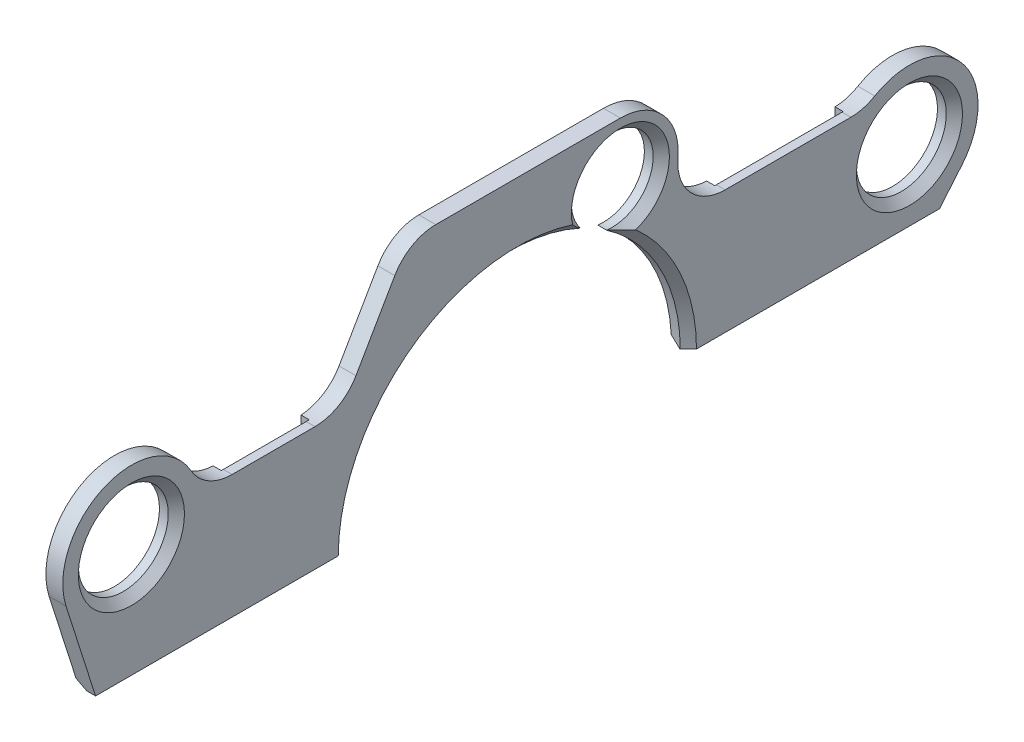
from build123d import *

# Parameters (mm, degrees)
BOSS_EXTRUDE1_DEPTH     = 12.5
CUT_EXTRUDE1_DEPTH      = 768.828594154
CUT_EXTRUDE1_DEPTH_BACK = 768.828594154
SKETCH2_R               = 60.5
SKETCH2_R_2             = 66.5
FILLET1_R               = 70
CHAMFER1_SIZE           = 12
CHAMFER2_SIZE           = 12
CUT_EXTRUDE2_DEPTH      = 65
CUT_EXTRUDE3_DEPTH      = 95


with BuildPart() as part:
    # Sketch1 → Boss-Extrude1 (new, symmetric)
    with BuildSketch(Plane(origin=(0, 0, 0), x_dir=(0, 0, -1), z_dir=(1, 0, 0))):
        with BuildLine():
            Line((-161.139129372, 353.5), (152.4, 353.5))
            ThreePointArc((152.4, 353.5), (215.520549571, 325.671884154), (237.552772458, 260.302250804))
            ThreePointArc((237.552772458, 260.302250804), (255.590849676, 206.783252739), (307.268492599, 184))
            Line((307.268492599, 184), (515.051943832, 184))
            ThreePointArc((515.051943832, 184), (651.90709321, 177.635326105), (657.753510977, 40.757057617))
            Line((657.753510977, 40.757057617), (624.56119852, 1.2))
            Line((624.56119852, 1.2), (252.997154134, 1.2))
            ThreePointArc((252.997154134, 1.2), (0, 253), (-252.997154134, 1.2))
            Line((-252.997154134, 1.2), (-624, 1.2))
            Line((-624, 1.2), (-667.696816027, 138.145895408))
            ThreePointArc((-667.696816027, 138.145895408), (-594.001115997, 267.859489493), (-470.614493078, 184))
            Line((-470.614493078, 184), (-259, 184))
            Line((-259, 184), (-161.139129372, 353.5))
        make_face()
    extrude(amount=BOSS_EXTRUDE1_DEPTH, both=True)

    # Sketch2 → Cut-Extrude1 (cut, two sides: drawn at the far end of the back side and taken through both)
    with BuildSketch(Plane(origin=(0, 0, 0), x_dir=(0, 0, -1), z_dir=(1, 0, 0)).offset(-CUT_EXTRUDE1_DEPTH_BACK)):
        with Locations((152.4, 268)):
            Circle(SKETCH2_R)
        with Locations((-571, 169)):
            Circle(SKETCH2_R_2)
        with Locations((580, 106)):
            Circle(SKETCH2_R_2)
    extrude(amount=CUT_EXTRUDE1_DEPTH + CUT_EXTRUDE1_DEPTH_BACK, mode=Mode.SUBTRACT)

    # Fillet1
    fillet1_edges = [part.edges().sort_by_distance(p)[0] for p in [
        (0, 184, 470.614493078),
        (0, 184, 259),
        (0, 353.5, 161.139129372),
        (0, 184, -515.051943832),
    ]]
    fillet(fillet1_edges, radius=FILLET1_R)

    # Chamfer1
    chamfer1_edges = [part.edges().sort_by_distance(p)[0] for p in [
        (12.5, 213.213707904, 136.194400626),
        (12.5, 118.018425376, -223.787066811),
        (12.5, 320.591390839, -182.306447626),
        (12.5, 169, 637.5),
        (12.5, 106, -513.5),
    ]]
    chamfer(chamfer1_edges, length=CHAMFER1_SIZE)

    # Chamfer2
    chamfer2_edges = [part.edges().sort_by_distance(p)[0] for p in [
        (-12.5, 1.2, -438.779176327),
        (-12.5, 1.2, 438.498577067),
    ]]
    chamfer(chamfer2_edges, length=CHAMFER2_SIZE)

    # Sketch3 → Cut-Extrude2 (cut, symmetric)
    with BuildSketch(Plane.XY.offset(360)):
        Polygon((5.5, 190), (-12.5, 172), (-12.5, 190), align=None)
    extrude(amount=CUT_EXTRUDE2_DEPTH, both=True, mode=Mode.SUBTRACT)

    # Sketch4 → Cut-Extrude3 (cut, symmetric)
    with BuildSketch(Plane.XY.offset(-400)):
        Polygon((-12.5, 172), (5.5, 190), (-12.5, 190), align=None)
    extrude(amount=CUT_EXTRUDE3_DEPTH, both=True, mode=Mode.SUBTRACT)


solid = part.part
